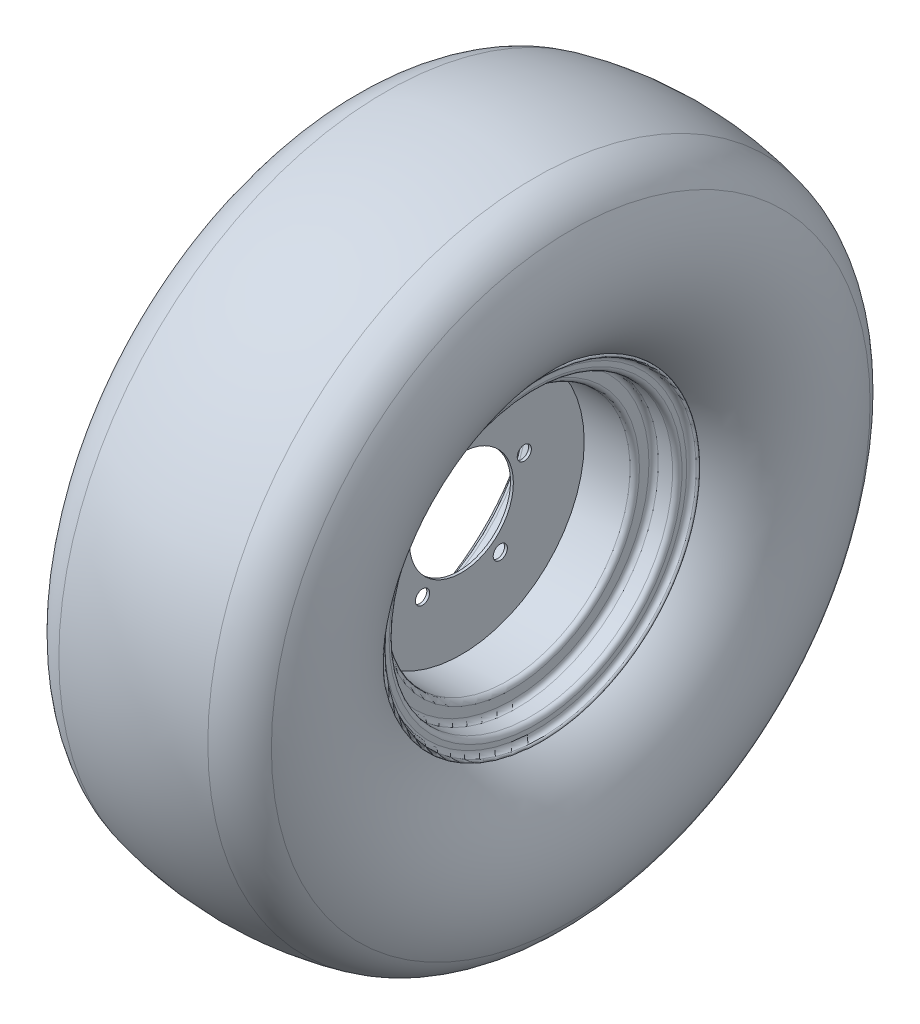
from build123d import *

# Parameters (mm, degrees)
SKETCH_2_R      = 130
SKETCH_2_R_2    = 55
SKETCH_2_R_3    = 7.5
EXTRUDE_1_DEPTH = 1.5


with BuildPart() as part:
    # 草图1 → 旋转1 (revolve)
    with BuildSketch(Plane.XY, mode=Mode.PRIVATE) as revolve_1_sk:
        with BuildLine():
            Line((-50, 0), (50, 0))
            ThreePointArc((50, 0), (53.535533906, -1.464466094), (55, -5))
            Line((55, -5), (55, -15))
            ThreePointArc((55, -15), (56.464466094, -18.535533906), (60, -20))
            Line((60, -20), (75, -20))
            ThreePointArc((75, -20), (78.535533906, -21.464466094), (80, -25))
            Line((80, -25), (80, -30))
            ThreePointArc((80, -30), (81.464466094, -33.535533906), (85, -35))
            ThreePointArc((85, -35), (86.5, -36.5), (85, -38))
            ThreePointArc((85, -38), (79.343145751, -35.656854249), (77, -30))
            Line((77, -30), (77, -25))
            ThreePointArc((77, -25), (76.414213562, -23.585786438), (75, -23))
            Line((75, -23), (60, -23))
            ThreePointArc((60, -23), (54.343145751, -20.656854249), (52, -15))
            Line((52, -15), (52, -5))
            ThreePointArc((52, -5), (51.414213562, -3.585786438), (50, -3))
            Line((50, -3), (-50, -3))
            ThreePointArc((-50, -3), (-51.414213562, -3.585786438), (-52, -5))
            Line((-52, -5), (-52, -15))
            ThreePointArc((-52, -15), (-54.343145751, -20.656854249), (-60, -23))
            Line((-60, -23), (-75, -23))
            ThreePointArc((-75, -23), (-76.414213562, -23.585786438), (-77, -25))
            Line((-77, -25), (-77, -30))
            ThreePointArc((-77, -30), (-79.343145751, -35.656854249), (-85, -38))
            ThreePointArc((-85, -38), (-86.5, -36.5), (-85, -35))
            ThreePointArc((-85, -35), (-81.464466094, -33.535533906), (-80, -30))
            Line((-80, -30), (-80, -25))
            ThreePointArc((-80, -25), (-78.535533906, -21.464466094), (-75, -20))
            Line((-75, -20), (-60, -20))
            ThreePointArc((-60, -20), (-56.464466094, -18.535533906), (-55, -15))
            Line((-55, -15), (-55, -5))
            ThreePointArc((-55, -5), (-53.535533906, -1.464466094), (-50, 0))
        make_face()
    revolve(revolve_1_sk.sketch.rotate(Axis((-65.404917461, 130, 0), (1, 0, 0)), 270), axis=Axis((-65.404917461, 130, 0), (1, 0, 0)))



with BuildPart() as body_2:
    # 草图2 → 凸台-拉伸1 (new, symmetric)
    with BuildSketch(Plane(origin=(0, 0, 0), x_dir=(0, 0, -1), z_dir=(1, 0, 0))):
        with Locations(Location((0, 130, 0), (0, 0, 180))):
            Circle(SKETCH_2_R)
        with Locations((0, 130)):
            Circle(SKETCH_2_R_2, mode=Mode.SUBTRACT)
        with Locations((0, 200)):
            Circle(SKETCH_2_R_3, mode=Mode.SUBTRACT)
        with Locations((66.573956141, 151.631189606)):
            Circle(SKETCH_2_R_3, mode=Mode.SUBTRACT)
        with Locations((41.14496766, 73.368810394)):
            Circle(SKETCH_2_R_3, mode=Mode.SUBTRACT)
        with Locations((-41.14496766, 73.368810394)):
            Circle(SKETCH_2_R_3, mode=Mode.SUBTRACT)
        with Locations((-66.573956141, 151.631189606)):
            Circle(SKETCH_2_R_3, mode=Mode.SUBTRACT)
    extrude(amount=EXTRUDE_1_DEPTH, both=True)


with BuildPart() as part_1:
    add(part.part)

    add(body_2.part)  # 旋转2 merges body 2
    # 草图3 → 旋转2 (revolve)
    with BuildSketch(Plane.XY, mode=Mode.PRIVATE) as revolve_2_sk:
        with BuildLine():
            Line((-77, 285), (-77, 290))
            ThreePointArc((-77, 290), (-79.343145751, 295.656854249), (-85, 298))
            ThreePointArc((-85, 298), (-129.406133001, 366.30461016), (-117.217363461, 446.858060205))
            ThreePointArc((-117.217363461, 446.858060205), (-101.044267901, 465.317950684), (-78.832909756, 475.757881041))
            ThreePointArc((-78.832909756, 475.757881041), (0, 485), (78.832909756, 475.757881041))
            ThreePointArc((78.832909756, 475.757881041), (101.044267901, 465.317950684), (117.217363461, 446.858060205))
            ThreePointArc((117.217363461, 446.858060205), (129.406133001, 366.30461016), (85, 298))
            ThreePointArc((85, 298), (79.343145751, 295.656854249), (77, 290))
            Line((77, 290), (77, 285))
            ThreePointArc((77, 285), (76.414213562, 283.585786438), (75, 283))
            Line((75, 283), (60, 283))
            ThreePointArc((60, 283), (54.343145751, 280.656854249), (52, 275))
            Line((52, 275), (52, 265))
            ThreePointArc((52, 265), (51.414213562, 263.585786438), (50, 263))
            Line((50, 263), (-50, 263))
            ThreePointArc((-50, 263), (-51.414213562, 263.585786438), (-52, 265))
            Line((-52, 265), (-52, 275))
            ThreePointArc((-52, 275), (-54.343145751, 280.656854249), (-60, 283))
            Line((-60, 283), (-75, 283))
            ThreePointArc((-75, 283), (-76.414213562, 283.585786438), (-77, 285))
        make_face()
    revolve(revolve_2_sk.sketch.rotate(Axis((50, 130, 0), (-1, 0, 0)), 90), axis=Axis((50, 130, 0), (-1, 0, 0)))


solid = part_1.part
